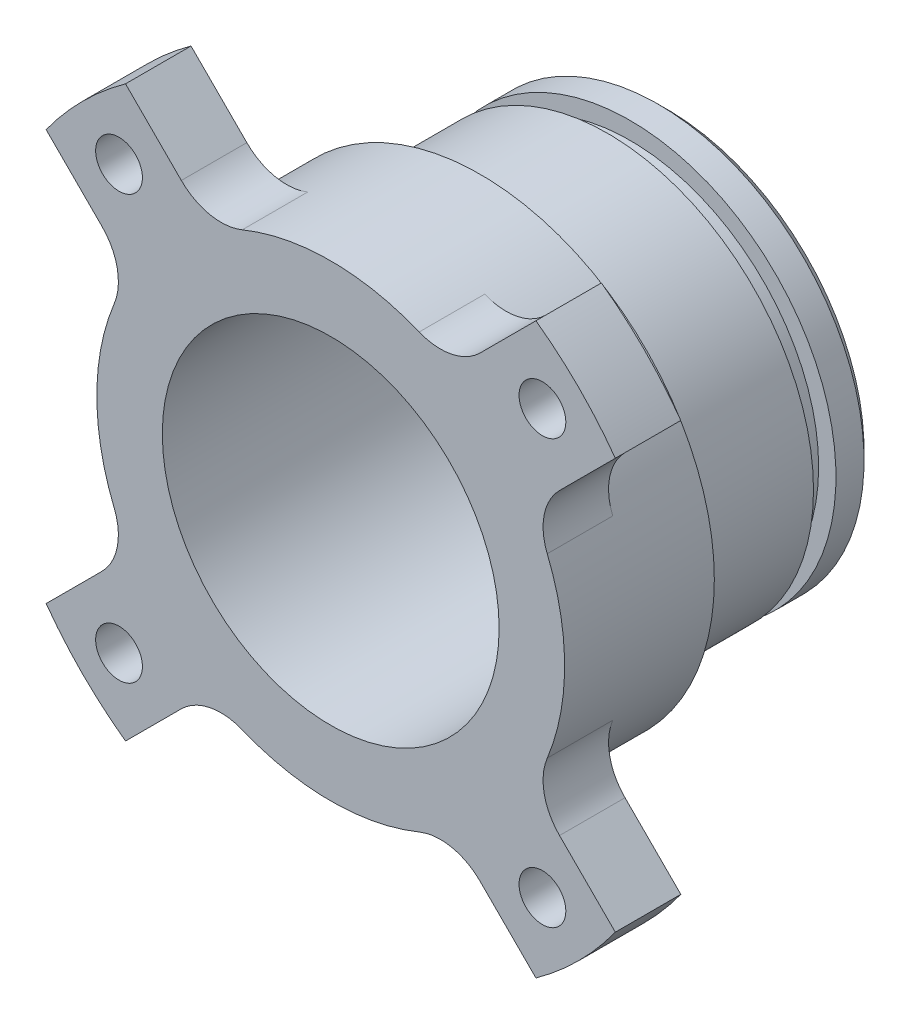
SolidWorks part; units mm, degrees
material "6061 合金"
ref_plane "前视基准面" through (0, 0, 0) normal (0, 0, 1) x (1, 0, 0)
ref_plane "上视基准面" through (0, 0, 0) normal (0, 1, 0) x (1, 0, 0)
ref_plane "右视基准面" through (0, 0, 0) normal (1, 0, 0) x (0, 0, -1)
other "Configuration Table"
sketch "草图1" plane through (0, 0, 0) normal (0, 0, 1) x (1, 0, 0)
  circle A0 centre (0, 0) radius 11
  circle A1 centre (0, 0) radius 9
  dimension "D1" = 22
  dimension "D2" = 18
extrude "凸台-拉伸1" add sketch "草图1" along normal blind 6.8
sketch "草图2" plane through (0, 0, 6.8) normal (0, 0, 1) x (1, 0, 0)
  circle A0 centre (0, 0) radius 9
  circle A1 centre (0, 0) radius 12.5
  dimension "D1" = 25
  dimension "D2" = 18
extrude "凸台-拉伸2" add sketch "草图2" along normal blind 8
sketch "草图4" plane through (0, 0, 14.8) normal (0, 0, 1) x (1, 0, 0)
  circle A1 centre (0, 0) radius 9 construction
  circle A2 centre (0, 0) radius 12.5
  circle A3 centre (0, 0) radius 12.5
  circle A4 centre (0, 0) radius 9
  dimension "D1" = 0
extrude "凸台-拉伸3" add sketch "草图4" along normal blind 5
sketch "草图8" plane through (0, 0, 19.8) normal (0, 0, 1) x (1, 0, 0)
  circle A0 centre (0, 0) radius 12.5 construction
  circle A1 centre (0, 0) radius 12.5
  circle A2 centre (0, 0) radius 9 construction
  circle A3 centre (0, 0) radius 9
extrude "切除-拉伸1" cut sketch "草图8" against normal blind 5
sketch "草图5" plane through (0, 0, 14.8) normal (0, 0, 1) x (1, 0, 0)
  line L0 (0, 0) -> (16, 0) construction
  line L1 (16, 2.5) -> (12.2474, 2.5)
  line L2 (16, -2.5) -> (12.2474, -2.5)
  arc A0 (16, -2.5) -> (16, 2.5) centre (16, 0) ccw
  circle A1 centre (16, 0) radius 1.5 construction
  circle A4 centre (0, 0) radius 12.5 construction
  arc A5 (12.2474, -2.5) -> (12.2474, 2.5) centre (0, 0) ccw
  dimension "D1" = 5
  dimension "D2" = 3
  dimension "D3" = 16
chamfer "倒角1" [suppressed] distance 0.5 angle 45
sketch "草图9" plane through (0, 0, 14.8) normal (0, 0, 1) x (1, 0, 0)
  line L0 (0, 0) -> (16, 0) construction
  line L1 (0, 0) -> (11.3137, 11.3137) construction
  line L2 (10.9661, 15.2088) -> (6.4592, 10.7018)
  line L3 (15.2088, 10.9661) -> (10.7018, 6.4592)
  line L4 (15.2088, -10.9661) -> (10.7018, -6.4592)
  line L5 (10.9661, -15.2088) -> (6.4592, -10.7018)
  line L6 (-10.9661, -15.2088) -> (-6.4592, -10.7018)
  line L7 (-15.2088, -10.9661) -> (-10.7018, -6.4592)
  line L8 (-15.2088, 10.9661) -> (-10.7018, 6.4592)
  line L9 (-10.9661, 15.2088) -> (-6.4592, 10.7018)
  circle A0 centre (0, 0) radius 16 construction
  circle A1 centre (11.3137, 11.3137) radius 1.5 construction
  arc A2 (15.2088, 10.9661) -> (10.9661, 15.2088) centre (0, 0) ccw
  arc A3 (10.7018, 6.4592) -> (6.4592, 10.7018) centre (0, 0) ccw
  arc A4 (10.9661, -15.2088) -> (15.2088, -10.9661) centre (0, 0) ccw
  circle A5 centre (11.3137, -11.3137) radius 1.5 construction
  arc A6 (6.4592, -10.7018) -> (10.7018, -6.4592) centre (0, 0) ccw
  arc A7 (-15.2088, -10.9661) -> (-10.9661, -15.2088) centre (0, 0) ccw
  circle A8 centre (-11.3137, -11.3137) radius 1.5 construction
  arc A9 (-10.7018, -6.4592) -> (-6.4592, -10.7018) centre (0, 0) ccw
  arc A10 (-10.9661, 15.2088) -> (-15.2088, 10.9661) centre (0, 0) ccw
  circle A11 centre (-11.3137, 11.3137) radius 1.5 construction
  arc A12 (-6.4592, 10.7018) -> (-10.7018, 6.4592) centre (0, 0) ccw
  point P31 (0, 0)
  dimension "D1" = 32
  dimension "D3" = 3
  dimension "D4" = 37.5
  dimension "D5" = 25
  dimension "D2" = 45
  dimension "D6" = 3
  dimension "D7" = 4
extrude "凸台-拉伸4" add sketch "草图9" against normal blind 3.5
hole_wizard "M3 螺纹孔1" positions "草图15" profile "草图11" tap size "M3" standard "GB" end condition through all
sketch "草图15" plane through (0, 0, 14.8) normal (0, 0, 1) x (1, 0, 0)
  point P0 (-11.3137, 11.3137)
  point P3 (11.3137, 11.3137)
  point P6 (11.3137, -11.3137)
  point P9 (-11.3137, -11.3137)
sketch "草图11" plane through (-11.3137, 11.3137, 14.8) normal (1, 0, 0) x (0, -1, 0)
  line L0 (0, 0) -> (0, 14.8)
  line L1 (0, 14.8) -> (1.25, 14.8)
  line L2 (1.25, 14.8) -> (1.25, 0)
  line L5 (1.25, 0) -> (0, 0)
  line L11 (0, -6.35) -> (0, 107.95) construction
  dimension "通孔螺纹孔钻头直径" = 2.5
  dimension "通孔螺纹孔钻头深度" = 14.8
cosmetic thread "孔螺蚊线1"
cosmetic thread "孔螺蚊线2"
cosmetic thread "孔螺蚊线3"
cosmetic thread "孔螺蚊线4"
fillet "圆角1" radius 3 8 edges at (-10.7018, 6.4592, 13.05) (-10.7018, -6.4592, 13.05) (-6.4592, -10.7018, 13.05) (6.4592, -10.7018, 13.05) (10.7018, -6.4592, 13.05) (10.7018, 6.4592, 13.05) (6.4592, 10.7018, 13.05) (-6.4592, 10.7018, 13.05)
sketch "草图13" plane through (0, 0, 0) normal (0, 0, -1) x (-1, 0, 0)
  circle A0 centre (0, 0) radius 10.075
  circle A1 centre (0, 0) radius 9
  dimension "D1" = 20.15
  dimension "D2" = 18
extrude "凸台-拉伸5" add sketch "草图13" along normal blind 1.2
sketch "草图14" plane through (0, 0, -1.2) normal (0, 0, -1) x (-1, 0, 0)
  circle A0 centre (0, 0) radius 9
  circle A1 centre (0, 0) radius 11
  dimension "D1" = 18
  dimension "D2" = 22
extrude "凸台-拉伸6" add sketch "草图14" along normal blind 2
chamfer "倒角2" distance 0.5 angle 45 1 edges at (-11, 0, -3.2)
